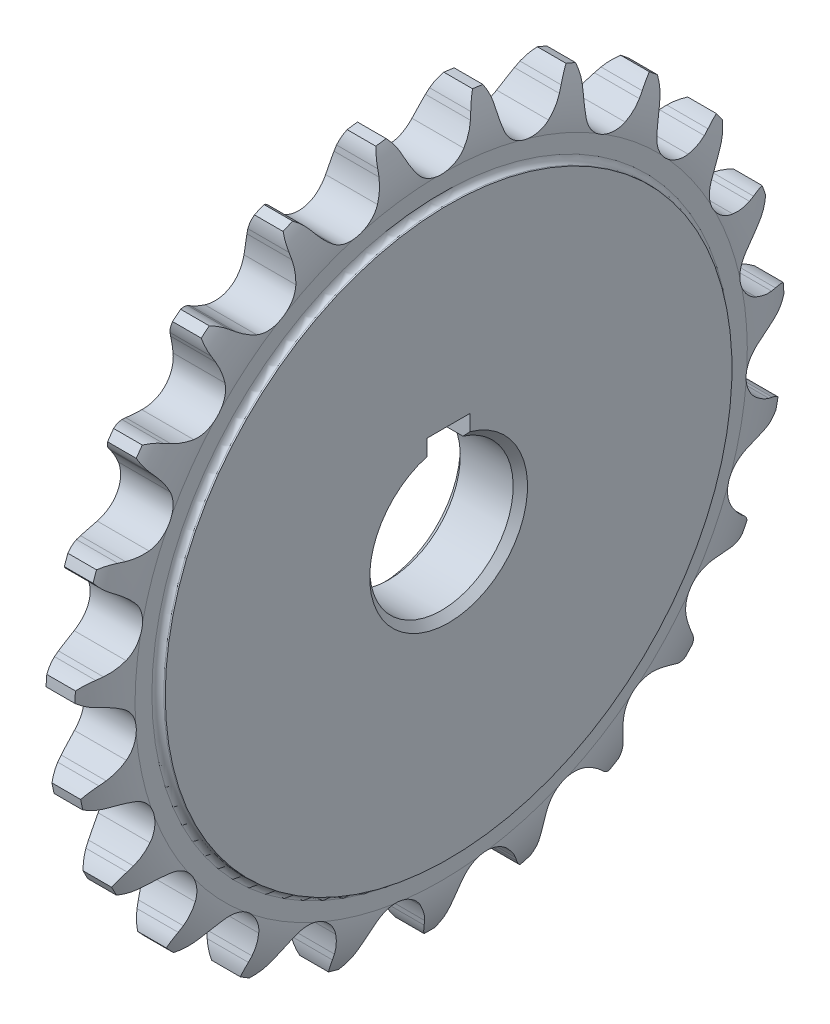
SolidWorks part; units mm, degrees
ref_plane "前视基准面" through (0, 0, 0) normal (0, 0, 1) x (1, 0, 0)
ref_plane "上视基准面" through (0, 0, 0) normal (0, 1, 0) x (1, 0, 0)
ref_plane "右视基准面" through (0, 0, 0) normal (1, 0, 0) x (0, 0, -1)
sketch "草图1" plane through (0, 0, 0) normal (0, 0, 1) x (1, 0, 0)
  line L0 (-6.35, 0) -> (6.35, 0) construction
  line L1 (-4.6852, 10) -> (-4.6852, 39.5)
  line L2 (-4.6852, 39.5) -> (-4.4782, 39.5)
  line L3 (-3.6502, 40.3279) -> (-3.6502, 42.674)
  line L4 (-1.9992, 49.5) -> (1.9992, 49.5)
  line L5 (3.6502, 42.674) -> (3.6502, 40.3279)
  line L6 (4.4782, 39.5) -> (4.6852, 39.5)
  line L7 (4.6852, 39.5) -> (4.6852, 10)
  line L8 (4.6852, 10) -> (-4.6852, 10)
  line L9 (0, 0) -> (0, 49.5) construction
  line L10 (-3.1938, 46.634) -> (3.1938, 46.634) construction
  line L11 (-3.1938, -46.634) -> (3.1938, -46.634) construction
  line L12 (6.35, 0) -> (29.35, 0) construction
  line L13 (-3.6502, 42.674) -> (3.7984, 42.674) construction
  line L14 (-3.6502, -42.674) -> (3.7984, -42.674) construction
  line L15 (29.35, 0) -> (37.27, 0) construction
  line L16 (37.27, 0) -> (49.34, 0) construction
  line L17 (49.34, 0) -> (57.19, 0) construction
  line L18 (57.19, 0) -> (71.57, 0) construction
  arc A0 (-1.9992, 49.5) -> (-3.6502, 42.674) centre (9.0381, 43.2177) ccw
  arc A1 (1.9992, 49.5) -> (3.6502, 42.674) centre (-9.0381, 43.2177) cw
  arc A2 (3.6502, 40.3279) -> (4.4782, 39.5) centre (4.4782, 40.3279) ccw
  arc A3 (-4.4782, 39.5) -> (-3.6502, 40.3279) centre (-4.4782, 40.3279) ccw
  point P30 (3.6502, 39.5)
  point P33 (-3.6502, 39.5)
  dimension "D1" = 3.174
  dimension "rx" = 12.7
  dimension "D3" = 0.8279
  dimension "d" = 93.2681
  dimension "p" = 12.7
  dimension "z" = 23
  dimension "da" = 99
  dimension "df" = 85.3481
  dimension "dr" = 7.92
  dimension "dk" = 20
  dimension "dg" = 79
  dimension "h" = 12.07
  dimension "bf1" = 7.3005
  dimension "b1" = 7.85
  dimension "ba" = 1.651
  dimension "D2" = 1.0349
  dimension "pt" = 14.38
revolve "旋转1" add sketch "草图1" angle 360 about L0
sketch "草图2" plane through (0, 0, 0) normal (1, 0, 0) x (0, 0, -1)
  line L0 (0, 0) -> (0, 49.5) construction
  line L1 (0, 0) -> (-6.7402, 49.039) construction
  line L2 (0, 0) -> (-13.3549, 47.6644) construction
  line L3 (3.1924, 44.1748) -> (7.0277, 41.2203) construction
  line L4 (4.5887, 46.6103) -> (-5.0194, 50.5007) construction
  line L5 (0, 0) -> (6.7402, 49.039) construction
  line L6 (4.5887, 46.6103) -> (4.8997, 47.3783)
  line L7 (-4.5887, 46.6103) -> (-4.8997, 47.3783)
  circle A0 centre (0, 0) radius 49.5 construction
  arc A1 (3.1924, 44.1748) -> (-3.1924, 44.1748) centre (0, 46.634) cw
  arc A2 (3.1924, 44.1748) -> (4.5887, 46.6103) centre (-5.0194, 50.5007) ccw
  arc A3 (6.0185, 49.1328) -> (4.8997, 47.3783) centre (10.2001, 45.2321) ccw
  arc A4 (-3.1924, 44.1748) -> (-4.5887, 46.6103) centre (5.0194, 50.5007) cw
  arc A5 (-6.0185, 49.1328) -> (-4.8997, 47.3783) centre (-10.2001, 45.2321) cw
  arc A7 (6.0185, 49.1328) -> (-6.0185, 49.1328) centre (0, 0) ccw
  dimension "r1" = 4.0298
  dimension "r3" = 5.7185
  dimension "D1" = 15.652
  dimension "D2" = 7.826
  dimension "α/2" = 52.391
  dimension "M" = 5.0194
  dimension "T" = 3.8666
  dimension "β" = 15.565
  dimension "γ/2" = 14.217
  dimension "bc" = 0.8285
extrude "切除-拉伸1" cut sketch "草图2" against normal mid plane 9.3703
pattern_circular "阵列(圆周)1" count 23 over 360 about axis through (0, 0, 0) along (1, 0, 0) of "切除-拉伸1"
sketch "草图3" plane through (0, 0, 0) normal (0, 0, 1) x (1, 0, 0)
  line L0 (4.6852, 10) -> (10.3148, 10)
  line L3 (10.3148, 10) -> (10.3148, 19.066)
  line L4 (10.3148, 19.066) -> (4.6852, 19.066)
  line L5 (4.6852, 19.066) -> (4.6852, 10)
  line L6 (0, 0) -> (4.8, 0) construction
  line L8 (-4.6852, 39.5) -> (-4.6852, -39.5) construction
  dimension "h" = 9.066
  dimension "K" = 4.8
  dimension "L" = 15
revolve "旋转2" [suppressed] add sketch "草图3" angle 360 about L6
sketch "草图4" plane through (-4.6852, 0, 0) normal (-1, 0, 0) x (0, 0, 1)
  line L1 (-3, 9.5394) -> (3, 9.5394)
  line L2 (-3, 9.5394) -> (-3, 12.8)
  line L3 (-3, 12.8) -> (3, 12.8)
  line L4 (3, 9.5394) -> (3, 12.8)
  circle A0 centre (0, 0) radius 10 construction
  point P6 (0.2, 12.8)
  dimension "D1" = 12.8
  dimension "键槽宽度" = 6
  dimension "t1" = 2.8
extrude "切除-拉伸2" cut sketch "草图4" against normal through all
chamfer "倒角1" distance 1 angle 45 1 edges at (-4.6852, -10, 0)
chamfer "倒角2" distance 1 angle 45 1 edges at (4.6852, -10, 0)
chamfer "倒角3" [suppressed] distance 1 angle 45
